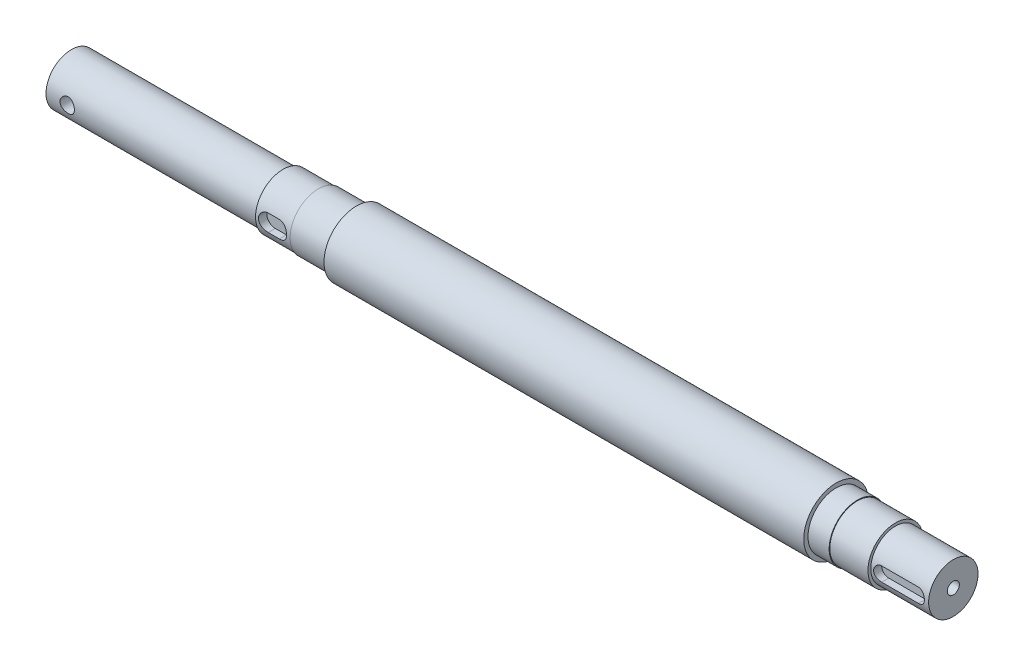
SolidWorks part; units mm, degrees
ref_plane "前视基准面" through (0, 0, 0) normal (0, 0, 1) x (1, 0, 0)
ref_plane "上视基准面" through (0, 0, 0) normal (0, 1, 0) x (1, 0, 0)
ref_plane "右视基准面" through (0, 0, 0) normal (1, 0, 0) x (0, 0, -1)
sketch "草图1" plane through (0, 0, 0) normal (1, 0, 0) x (0, 0, -1)
  circle A0 centre (0, 0) radius 23
extrude "凸台-拉伸1" add sketch "草图1" along normal blind 340
sketch "草图2" plane through (0, 0, 0) normal (-1, 0, 0) x (0, 0, 1)
  circle A0 centre (0, 0) radius 20
extrude "凸台-拉伸2" add sketch "草图2" along normal blind 27
sketch "草图3" plane through (-27, 0, 0) normal (-1, 0, 0) x (0, 0, 1)
  circle A0 centre (0, 0) radius 19.5
extrude "凸台-拉伸3" add sketch "草图3" along normal blind 25
sketch "草图4" plane through (340, 0, 0) normal (1, 0, 0) x (0, 0, -1)
  circle A0 centre (0, 0) radius 20
extrude "凸台-拉伸4" add sketch "草图4" along normal blind 15
sketch "草图5" plane through (355, 0, 0) normal (1, 0, 0) x (0, 0, -1)
  circle A0 centre (0, 0) radius 19.5
extrude "凸台-拉伸5" add sketch "草图5" along normal blind 27
sketch "草图6" plane through (382, 0, 0) normal (1, 0, 0) x (0, 0, -1)
  circle A0 centre (0, 0) radius 17.5
extrude "凸台-拉伸6" add sketch "草图6" along normal blind 41
ref_plane "基准面1" through (0, 0, 17.5) normal (0, 0, 1) x (1, 0, 0)
sketch "草图7" plane through (0, 0, 17.5) normal (0, 0, 1) x (1, 0, 0)
  line L0 (389, 0) -> (415, 0) construction
  line L1 (389, 5) -> (415, 5)
  line L2 (389, -5) -> (415, -5)
  line L3 (382, -17.5) -> (382, 17.5) construction
  arc A0 (389, 5) -> (389, -5) centre (389, 0) ccw
  arc A1 (415, -5) -> (415, 5) centre (415, 0) ccw
  point P3 (402, 0)
  dimension "D1" = 5
  dimension "D3" = 7
  dimension "D2" = 26
extrude "切除-拉伸1" cut sketch "草图7" against normal blind 5.73
sketch "草图8" plane through (-52, 0, 0) normal (-1, 0, 0) x (0, 0, 1)
  circle A0 centre (0, 0) radius 18
extrude "凸台-拉伸7" add sketch "草图8" along normal blind 150
ref_plane "基准面2" through (0, 0, 18) normal (0, 0, 1) x (1, 0, 0)
hole_wizard "M12 螺纹孔2" positions "草图13" profile "草图12" tap size "M12" standard "Iso"
sketch "草图13" plane through (0, 0, 18) normal (0, 0, 1) x (1, 0, 0)
  line L0 (-202, 18) -> (-202, -18) construction
  point P0 (-187, 0)
  dimension "D1" = 15
sketch "草图12" plane through (-187, 0, 18) normal (1, 0, 0) x (0, -1, 0)
  line L0 (0, 0) -> (0, 23.0644)
  line L1 (0, 23.0644) -> (5.1, 20)
  line L2 (5.1, 20) -> (5.1, 0)
  line L5 (5.1, 0) -> (0, 0)
  line L10 (0, 23.0644) -> (-5.1, 20) construction
  line L11 (0, -6.35) -> (0, 107.95) construction
  dimension "螺纹孔钻头直径" = 10.2
  dimension "螺纹孔钻头深度" = 20
  dimension "导头角度" = 118
cosmetic thread "孔螺蚊线2" parameters "D1"=20, "D2"=12
hole_wizard "M10 螺纹孔1" positions "草图17" profile "草图16" tap size "M10" standard "Iso"
sketch "草图17" plane through (423, 0, 0) normal (1, 0, 0) x (0, 0, -1)
  point P0 (0, 0)
sketch "草图16" plane through (423, 0, 0) normal (0, 1, 0) x (0, 0, -1)
  line L0 (0, 0) -> (0, 22.5537)
  line L1 (0, 22.5537) -> (4.25, 20)
  line L2 (4.25, 20) -> (4.25, 0)
  line L5 (4.25, 0) -> (0, 0)
  line L10 (0, 22.5537) -> (-4.25, 20) construction
  line L11 (0, -6.35) -> (0, 107.95) construction
  dimension "螺纹孔钻头直径" = 8.5
  dimension "螺纹孔钻头深度" = 20
  dimension "导头角度" = 118
cosmetic thread "孔螺蚊线3" parameters "D1"=20, "D2"=10
sketch "草图18" plane through (0, 0, 17.5) normal (0, 0, 1) x (1, 0, 0)
  line L0 (-36, 0) -> (-44, 0) construction
  line L1 (-36, -6) -> (-44, -6)
  line L2 (-36, 6) -> (-44, 6)
  line L3 (-27, 20) -> (-27, -20) construction
  arc A0 (-36, -6) -> (-36, 6) centre (-36, 0) ccw
  arc A1 (-44, 6) -> (-44, -6) centre (-44, 0) ccw
  point P3 (-40, 0)
  dimension "D1" = 8
  dimension "D2" = 6
  dimension "D3" = 9
extrude "切除-拉伸2" cut sketch "草图18" against normal blind 3.95 and the other way blind 5
